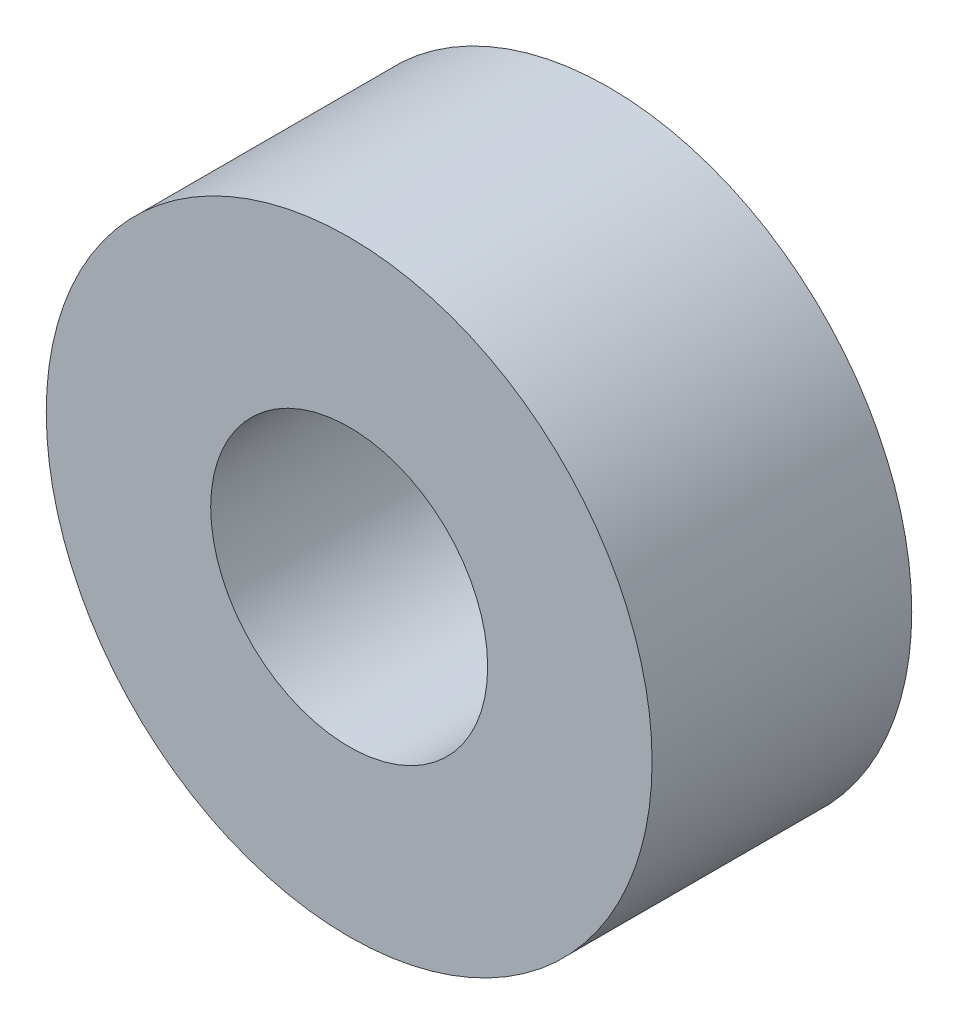
from build123d import *

# Parameters (mm, degrees)
SKETCH_1_R      = 17.5
SKETCH_1_R_2    = 8
EXTRUDE_1_DEPTH = 7.5


with BuildPart() as part:
    # 草图1 → 凸台-拉伸1 (new, symmetric)
    with BuildSketch(Plane.XY):
        Circle(SKETCH_1_R)
        Circle(SKETCH_1_R_2, mode=Mode.SUBTRACT)
    extrude(amount=EXTRUDE_1_DEPTH, both=True)


solid = part.part
